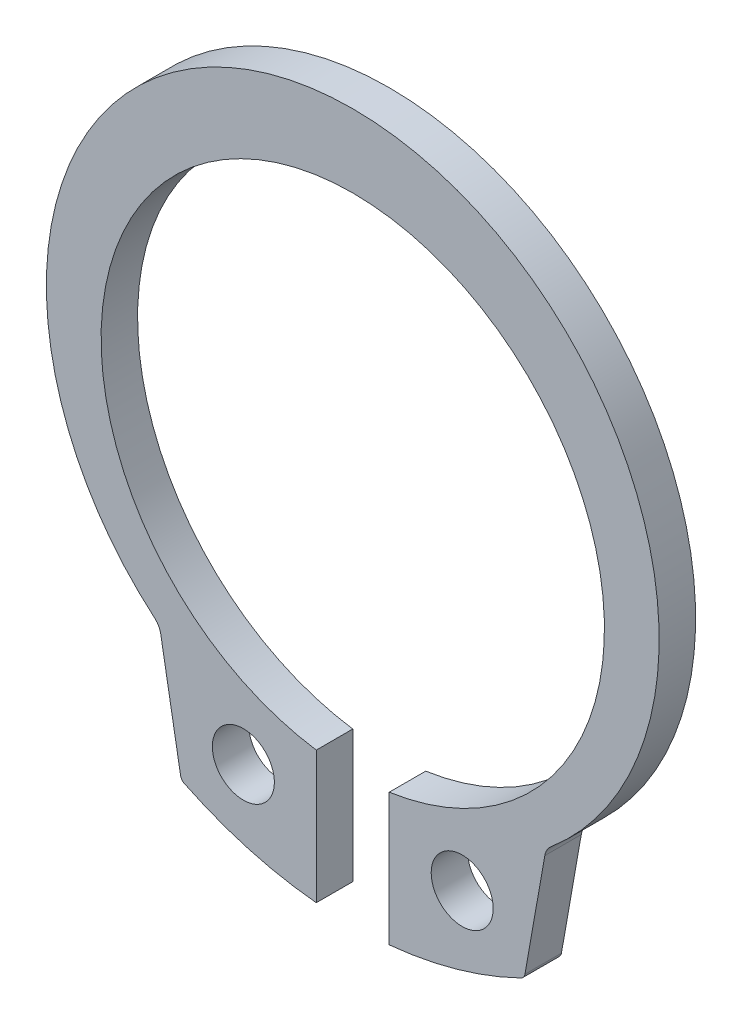
SolidWorks part; units mm, degrees
ref_plane "前视基准面" through (0, 0, 0) normal (0, 0, 1) x (1, 0, 0)
ref_plane "上视基准面" through (0, 0, 0) normal (0, 1, 0) x (1, 0, 0)
ref_plane "右视基准面" through (0, 0, 0) normal (1, 0, 0) x (0, 0, -1)
sketch "草图1" plane through (0, 0, 0) normal (0, 0, 1) x (1, 0, 0)
  line L0 (-5.2651, -6.7) -> (-4.7206, -9.7882)
  line L1 (-1, -10.9523) -> (-1, -7.3272)
  line L2 (1, -7.3272) -> (1, -10.9523)
  line L3 (4.7206, -9.7882) -> (5.2651, -6.7)
  circle A0 centre (3, -8.6664) radius 0.85
  circle A1 centre (-3, -8.6664) radius 0.85
  arc A2 (5.4341, -6.4055) -> (-5.4341, -6.4055) centre (0, 0) ccw
  arc A3 (-5.4341, -6.4055) -> (-5.2651, -6.7) centre (-5.7575, -6.7868) cw
  arc A4 (-4.7206, -9.7882) -> (-4.6115, -9.9332) centre (-4.5236, -9.7535) ccw
  arc A5 (-4.6115, -9.9332) -> (-1, -10.9523) centre (0, -0.5) ccw
  arc A6 (-1, -7.3272) -> (1, -7.3272) centre (0, -0.5) cw
  arc A7 (1, -10.9523) -> (4.6115, -9.9332) centre (0, -0.5) ccw
  arc A8 (4.6115, -9.9332) -> (4.7206, -9.7882) centre (4.5236, -9.7535) ccw
  arc A9 (5.2651, -6.7) -> (5.4341, -6.4055) centre (5.7575, -6.7868) cw
extrude "凸台-拉伸1" add sketch "草图1" against normal blind 1
